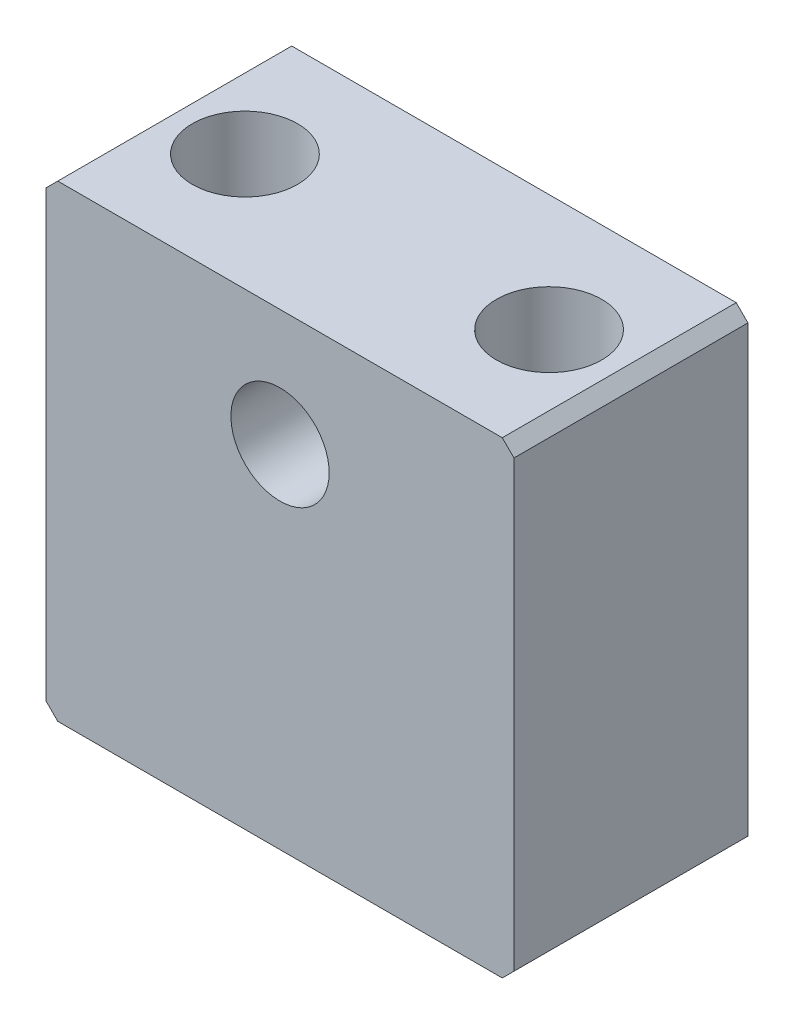
SolidWorks part; units mm, degrees
material "AL6061"
ref_plane "Front Plane" through (0, 0, 0) normal (0, 0, 1) x (1, 0, 0)
ref_plane "Top Plane" through (0, 0, 0) normal (0, 1, 0) x (1, 0, 0)
ref_plane "Right Plane" through (0, 0, 0) normal (1, 0, 0) x (0, 0, -1)
sketch "Sketch1" plane through (0, 0, 0) normal (0, 1, 0) x (1, 0, 0)
  line L1 (-10, -5) -> (10, -5)
  line L2 (-10, -5) -> (-10, 5)
  line L3 (-10, 5) -> (10, 5)
  line L4 (10, -5) -> (10, 5)
  line L5 (-10, -5) -> (10, 5) construction
  line L6 (-10, 5) -> (10, -5) construction
  point P0 (0, 0)
  dimension "D1" = 10
  dimension "D2" = 20
extrude "Boss-Extrude1" add sketch "Sketch1" along normal mid plane 20
hole_wizard "M5 Tapped Hole1" positions "Sketch2" profile "Sketch3" tap size "M5" standard "GB" end condition through all
sketch "Sketch2" plane through (0, 0, 5) normal (0, 0, 1) x (1, 0, 0)
  line L0 (0, 0) -> (0, 8.5694) construction
  line L1 (-10, 10) -> (10, 10) construction
  point P11 (0, 5)
  dimension "D1" = 5
sketch "Sketch3" plane through (0, 5, 5) normal (1, 0, 0) x (0, -1, 0)
  line L0 (0, 0) -> (0, 10)
  line L1 (0, 10) -> (2.1, 10)
  line L2 (2.1, 10) -> (2.1, 0)
  line L5 (2.1, 0) -> (0, 0)
  line L11 (0, -6.35) -> (0, 107.95) construction
  dimension "通孔螺纹孔钻头直径" = 4.2
  dimension "通孔螺纹孔钻头深度" = 10
cosmetic thread "Hole Thread1" parameters "D2"=5
hole_wizard "M4 Clearance Hole1" positions "Sketch6" profile "Sketch7" hole size "M4" standard "GB" end condition through all
sketch "Sketch6" plane through (0, 10, 0) normal (0, 1, 0) x (1, 0, 0)
  line L0 (0, 0) -> (0, 9.4241) construction
  line L3 (0, 0) -> (-16.3945, 0) construction
  point P12 (-6.5, 0)
  point P15 (6.5, 0)
  dimension "D1" = 13
sketch "Sketch7" plane through (6.5, 10, 0) normal (1, 0, 0) x (0, 0, 1)
  line L0 (0, 0) -> (0, 20)
  line L1 (0, 20) -> (2.25, 20)
  line L2 (2.25, 20) -> (2.25, 0)
  line L5 (2.25, 0) -> (0, 0)
  line L11 (0, -6.35) -> (0, 107.95) construction
  dimension "通孔孔直径" = 4.5
  dimension "通孔孔深度" = 20
chamfer "Chamfer1" distance 0.5 angle 45 4 edges at (10, 10, 0) (-10, 10, 0) (10, -10, 0) (-10, -10, 0)
